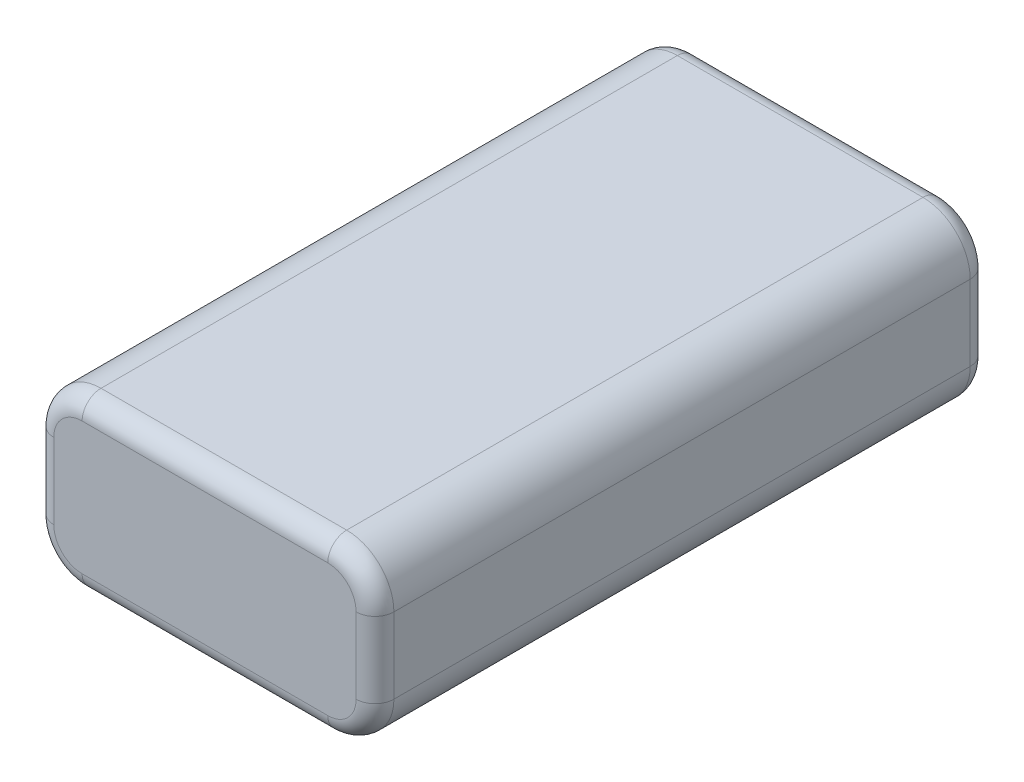
from build123d import *

# Parameters (mm, degrees)
SKETCH1_W           = 36
SKETCH1_H           = 18
BOSS_EXTRUDE1_DEPTH = 65
FILLET1_R           = 5
FILLET2_R           = 2


with BuildPart() as part:
    # Sketch1 → Boss-Extrude1 (new body)
    with BuildSketch(Plane.XY):
        Rectangle(SKETCH1_W, SKETCH1_H)
    extrude(amount=BOSS_EXTRUDE1_DEPTH)

    # Fillet1
    fillet1_edges = [part.edges().sort_by_distance(p)[0] for p in [
        (18, -9, 32.5),
        (-18, -9, 32.5),
        (-18, 9, 32.5),
        (18, 9, 32.5),
    ]]
    fillet(fillet1_edges, radius=FILLET1_R)

    # Fillet2
    fillet2_edges = [part.edges().sort_by_distance(p)[0] for p in [
        (0, -9, 0),
        (0, -9, 65),
        (18, 0, 0),
        (-18, 0, 0),
        (0, 9, 0),
        (16.535533906, 7.535533906, 0),
        (16.535533906, -7.535533906, 0),
        (-16.535533906, 7.535533906, 0),
        (-16.535533906, -7.535533906, 0),
        (-18, 0, 65),
        (18, 0, 65),
        (0, 9, 65),
        (16.535533906, 7.535533906, 65),
        (16.535533906, -7.535533906, 65),
        (-16.535533906, 7.535533906, 65),
        (-16.535533906, -7.535533906, 65),
    ]]
    fillet(fillet2_edges, radius=FILLET2_R)


solid = part.part
